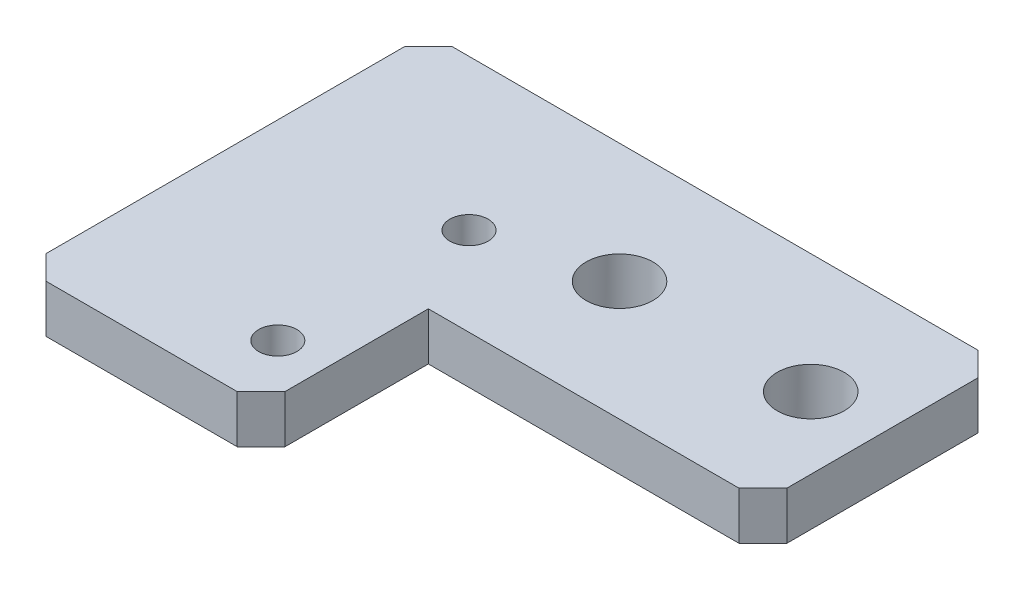
from build123d import *

# Parameters (mm, degrees)
SKETCH1_W             = 10
SKETCH1_H             = 17
BOSS_EXTRUDE1_DEPTH   = 2
SKETCH2_W             = 14
SKETCH2_H             = 10
BOSS_EXTRUDE2_DEPTH   = 2
SKETCH3_R             = 1.4
CUT_EXTRUDE1_DEPTH    = 10
CHAMFER1_SIZE         = 1
M2_TAPPED_HOLE1_D     = 1.6
M2_TAPPED_HOLE1_DEPTH = 5.2
M2_TAPPED_HOLE1_TIP   = 0.480688495


with BuildPart() as part:
    # Sketch1 → Boss-Extrude1 (new body)
    with BuildSketch(Plane(origin=(0, 0, 0), x_dir=(1, 0, 0), z_dir=(0, 1, 0))):
        with Locations((5, 8.5)):
            Rectangle(SKETCH1_W, SKETCH1_H)
    extrude(amount=BOSS_EXTRUDE1_DEPTH)

    # Sketch2 → Boss-Extrude2 (add)
    with BuildSketch(Plane(origin=(0, 2, 0), x_dir=(1, 0, 0), z_dir=(0, 1, 0))):
        with Locations((17, 12)):
            Rectangle(SKETCH2_W, SKETCH2_H)
    extrude(amount=-BOSS_EXTRUDE2_DEPTH)

    # Sketch3 → Cut-Extrude1 (cut)
    with BuildSketch(Plane(origin=(0, 2, 0), x_dir=(1, 0, 0), z_dir=(0, 1, 0))):
        with Locations(Location((21, 12, 0), (0, 0, 270))):
            Circle(SKETCH3_R)
        with Locations(Location((13, 12, 0), (0, 0, 270))):
            Circle(SKETCH3_R)
    extrude(amount=-CUT_EXTRUDE1_DEPTH, mode=Mode.SUBTRACT)

    # Chamfer1
    chamfer1_edges = [part.edges().sort_by_distance(p)[0] for p in [
        (0, 1, -17),
        (0, 1, 0),
        (10, 1, 0),
        (24, 1, -17),
        (24, 1, -7),
    ]]
    chamfer(chamfer1_edges, length=CHAMFER1_SIZE)

    # M2 Tapped Hole1
    with Locations(Plane(origin=(0, 2, 0), x_dir=(1, 0, 0), z_dir=(0, 1, 0))):
        with Locations((8, 10.7), (8, 2.7)):
            Hole(M2_TAPPED_HOLE1_D / 2, depth=M2_TAPPED_HOLE1_DEPTH)
            with Locations((0, 0, -(M2_TAPPED_HOLE1_DEPTH + M2_TAPPED_HOLE1_TIP / 2))):  # 118° drill point
                Cone(0, M2_TAPPED_HOLE1_D / 2, M2_TAPPED_HOLE1_TIP, mode=Mode.SUBTRACT)


solid = part.part
